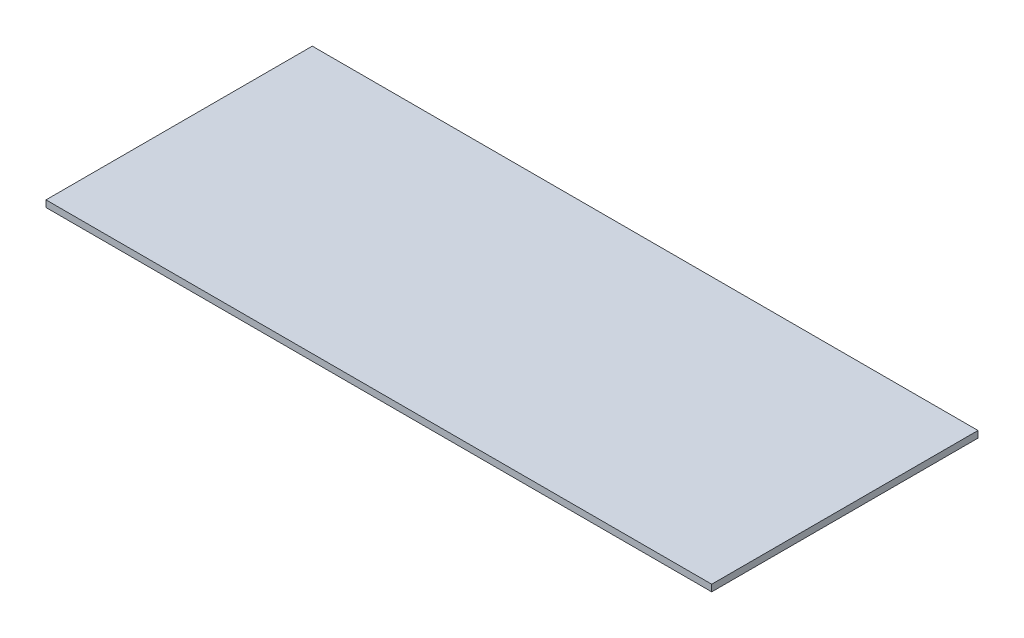
SolidWorks part; units mm, degrees
material "A3"
ref_plane "前视基准面" through (0, 0, 0) normal (0, 0, 1) x (1, 0, 0)
ref_plane "上视基准面" through (0, 0, 0) normal (0, 1, 0) x (1, 0, 0)
ref_plane "右视基准面" through (0, 0, 0) normal (1, 0, 0) x (0, 0, -1)
sketch "草图1" plane through (0, 0, 0) normal (0, 1, 0) x (1, 0, 0)
  line L1 (-50, -20) -> (50, -20)
  line L2 (-50, -20) -> (-50, 20)
  line L3 (-50, 20) -> (50, 20)
  line L4 (50, -20) -> (50, 20)
  line L5 (-50, -20) -> (50, 20) construction
  line L6 (-50, 20) -> (50, -20) construction
  point P0 (0, 0)
  dimension "D1" = 40
  dimension "D2" = 100
extrude "凸台-拉伸1" add sketch "草图1" along normal blind 1
